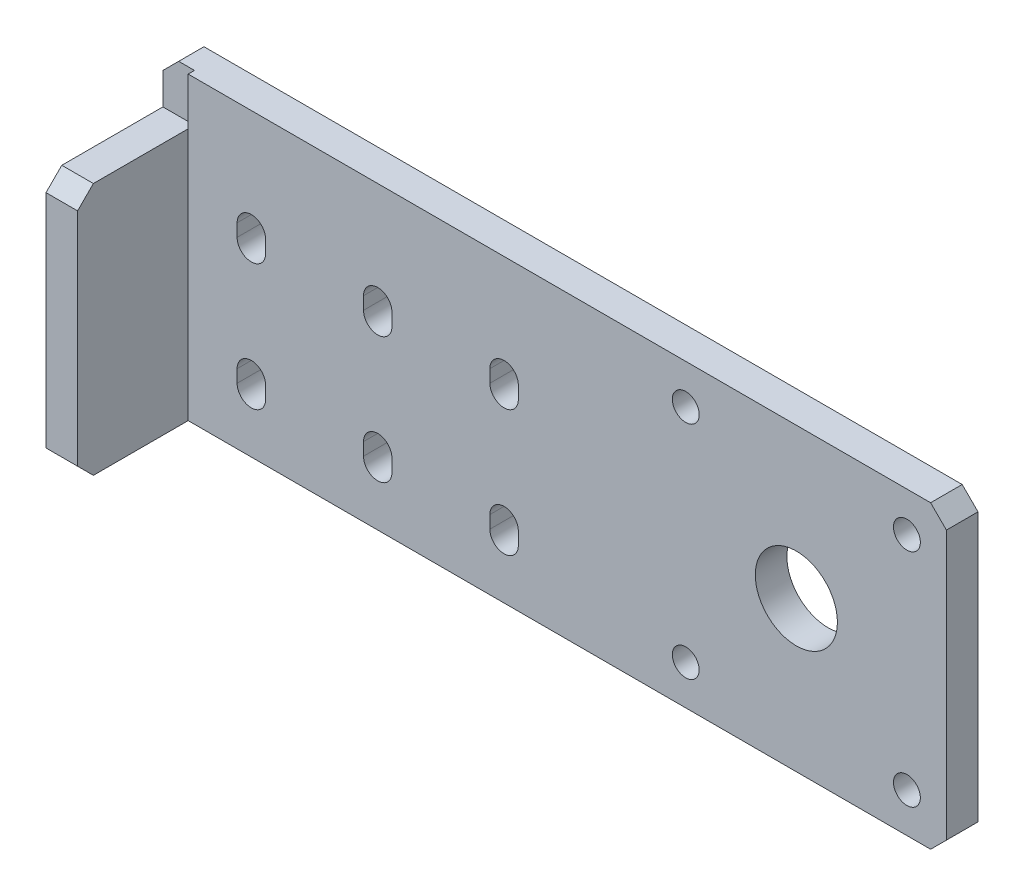
SolidWorks part; units mm, degrees
material "AISI 1045 钢，冷拔"
ref_plane "前视基准面" through (0, 0, 0) normal (0, 0, 1) x (1, 0, 0)
ref_plane "上视基准面" through (0, 0, 0) normal (0, 1, 0) x (1, 0, 0)
ref_plane "右视基准面" through (0, 0, 0) normal (1, 0, 0) x (0, 0, -1)
sketch "草图1" plane through (0, 0, 0) normal (0, 0, 1) x (1, 0, 0)
  line L1 (-125, 47.5) -> (125, 47.5)
  line L2 (-125, 47.5) -> (-125, -47.5)
  line L3 (-125, -47.5) -> (125, -47.5)
  line L4 (125, 47.5) -> (125, -47.5)
  line L5 (-125, 47.5) -> (125, -47.5) construction
  line L6 (-125, -47.5) -> (125, 47.5) construction
  point P0 (0, 0)
  dimension "D1" = 95
  dimension "D2" = 250
extrude "凸台-拉伸1" add sketch "草图1" along normal blind 10
sketch "草图3" plane through (0, 0, 10) normal (0, 0, 1) x (1, 0, 0)
  line L0 (-55, 17.5058) -> (-55, -69.5405) construction
  line L1 (125, -47.5) -> (125, 47.5) construction
  line L2 (-22.9727, -29.5) -> (-57.0867, -29.5) construction
  line L3 (-125, -47.5) -> (125, -47.5) construction
  line L4 (-55, -29.5) -> (-55, -25.5) construction
  line L5 (-59.5, -29.5) -> (-59.5, -25.5)
  line L6 (-50.5, -29.5) -> (-50.5, -25.5)
  arc A0 (-59.5, -29.5) -> (-50.5, -29.5) centre (-55, -29.5) ccw
  arc A1 (-50.5, -25.5) -> (-59.5, -25.5) centre (-55, -25.5) ccw
  point P10 (-55, -27.5)
  dimension "D4" = 4.5
  dimension "D1" = 180
  dimension "D2" = 18
  dimension "D3" = 4
extrude "切除-拉伸2" cut sketch "草图3" against normal through all
pattern_linear "阵列(线性)1" count 2 spacing 40 along (1, 0, 0) count 2 spacing 40 along (0, 1, 0) of "切除-拉伸2"
pattern_linear "阵列(线性)2" count 2 spacing 40 along (-1, 0, 0) count 2 spacing 40 along (0, 1, 0) of "切除-拉伸2"
sketch "草图10" plane through (0, 0, 10) normal (0, 0, 1) x (1, 0, 0)
  line L0 (24.75, 0) -> (-24.75, 0) construction
  line L1 (42.5, 35) -> (112.5, 35) construction
  line L2 (42.5, 35) -> (42.5, -35) construction
  line L3 (42.5, -35) -> (112.5, -35) construction
  line L4 (112.5, 35) -> (112.5, -35) construction
  line L5 (42.5, 35) -> (112.5, -35) construction
  line L6 (42.5, -35) -> (112.5, 35) construction
  line L7 (125, -47.5) -> (125, 47.5) construction
  point P0 (77.5, 0)
  dimension "D1" = 70
  dimension "D2" = 70
  dimension "D3" = 47.5
hole_wizard "M10 螺纹孔3" positions "3D草图3" profile "草图11" tap size "M10" standard "GB"
sketch3d "3D草图3"
  point P0 (42.5, 35, 10)
  point P3 (112.5, 35, 10)
  point P6 (112.5, -35, 10)
  point P9 (42.5, -35, 10)
sketch "草图11" plane through (42.5, 35, 10) normal (1, 0, 0) x (0, -1, 0)
  line L0 (0, 0) -> (0, 27.0537)
  line L1 (0, 27.0537) -> (4.25, 24.5)
  line L2 (4.25, 24.5) -> (4.25, 0)
  line L5 (4.25, 0) -> (0, 0)
  line L10 (0, 27.0537) -> (-4.25, 24.5) construction
  line L11 (0, -6.35) -> (0, 107.95) construction
  dimension "螺纹孔钻头直径" = 8.5
  dimension "螺纹孔钻头深度" = 24.5
  dimension "导头角度" = 118
cosmetic thread "孔螺蚊线9"
cosmetic thread "孔螺蚊线10"
cosmetic thread "孔螺蚊线11"
cosmetic thread "孔螺蚊线12"
sketch "草图12" plane through (0, 0, 10) normal (0, 0, 1) x (1, 0, 0)
  line L0 (42.5, 35) -> (112.5, -35) construction
  circle A0 centre (77.5, 0) radius 13
  dimension "D1" = 26
extrude "切除-拉伸5" cut sketch "草图12" against normal through all
sketch "草图13" plane through (0, 0, 0) normal (0, 0, -1) x (-1, 0, 0)
  line L0 (-45, -20) -> (-110, -20) construction
  line L1 (-110, -20) -> (-110, 20) construction
  line L2 (-110, 20) -> (-45, 20) construction
hole_wizard "M6 螺纹孔1" positions "3D草图4" profile "草图14" tap size "M6" standard "GB"
sketch3d "3D草图4"
  point P0 (45, -20, 0)
  point P3 (110, -20, 0)
  point P6 (110, 20, 0)
  point P9 (45, 20, 0)
sketch "草图14" plane through (45, -20, 0) normal (1, 0, 0) x (0, 1, 0)
  line L0 (0, 0) -> (0, 10)
  line L1 (0, 10) -> (2.5, 10)
  line L2 (2.5, 10) -> (2.5, 0)
  line L5 (2.5, 0) -> (0, 0)
  line L11 (0, -6.35) -> (0, 107.95) construction
  dimension "通孔螺纹孔钻头直径" = 5
  dimension "通孔螺纹孔钻头深度" = 10
cosmetic thread "孔螺蚊线17" [suppressed]
cosmetic thread "孔螺蚊线18" [suppressed]
cosmetic thread "孔螺蚊线19" [suppressed]
cosmetic thread "孔螺蚊线20" [suppressed]
sketch "草图15" plane through (-125, 0, 0) normal (-1, 0, 0) x (0, 0, 1)
  line L0 (5, -37.5) -> (5, -17.5) construction
  line L1 (5, -17.5) -> (5, 2.5) construction
  line L2 (5, 2.5) -> (5, 22.5) construction
hole_wizard "M6 螺纹孔2" positions "3D草图5" profile "草图16" tap size "M6" standard "GB"
sketch3d "3D草图5"
  point P0 (-125, -37.5, 5)
  point P3 (-125, -17.5, 5)
  point P6 (-125, 2.5, 5)
  point P9 (-125, 22.5, 5)
sketch "草图16" plane through (-125, -37.5, 5) normal (0, 1, 0) x (0, 0, 1)
  line L0 (0, 0) -> (0, 16.5022)
  line L1 (0, 16.5022) -> (2.5, 15)
  line L2 (2.5, 15) -> (2.5, 0)
  line L5 (2.5, 0) -> (0, 0)
  line L10 (0, 16.5022) -> (-2.5, 15) construction
  line L11 (0, -6.35) -> (0, 107.95) construction
  dimension "螺纹孔钻头直径" = 5
  dimension "螺纹孔钻头深度" = 15
  dimension "导头角度" = 118
cosmetic thread "孔螺蚊线21" [suppressed]
cosmetic thread "孔螺蚊线22" [suppressed]
cosmetic thread "孔螺蚊线23" [suppressed]
cosmetic thread "孔螺蚊线24" [suppressed]
sketch "草图18" plane through (0, -47.5, 0) normal (0, -1, 0) x (1, 0, 0)
  line L0 (12, 5) -> (47, 5) construction
  line L1 (47, 5) -> (82, 5) construction
  line L2 (82, 5) -> (117, 5) construction
  point P4 (64.5, 5)
hole_wizard "M4 螺纹孔1" positions "3D草图6" profile "草图19" tap size "M4" standard "GB"
sketch3d "3D草图6"
  point P0 (117, -47.5, 5)
  point P9 (12, -47.5, 5)
  point P12 (64.5, -47.5, 5)
sketch "草图19" plane through (117, -47.5, 5) normal (1, 0, 0) x (0, 0, -1)
  line L0 (0, 0) -> (0, 11.0914)
  line L1 (0, 11.0914) -> (1.65, 10.1)
  line L2 (1.65, 10.1) -> (1.65, 0)
  line L5 (1.65, 0) -> (0, 0)
  line L10 (0, 11.0914) -> (-1.65, 10.1) construction
  line L11 (0, -6.35) -> (0, 107.95) construction
  dimension "螺纹孔钻头直径" = 3.3
  dimension "螺纹孔钻头深度" = 10.1
  dimension "导头角度" = 118
cosmetic thread "孔螺蚊线25"
cosmetic thread "孔螺蚊线26"
cosmetic thread "孔螺蚊线28"
sketch "草图22" plane through (0, 0, 10) normal (0, 0, 1) x (1, 0, 0)
  line L0 (-125, -47.5) -> (125, -47.5) construction
  line L1 (-125, 47.5) -> (-115, 47.5)
  line L2 (-125, 47.5) -> (-125, -47.5)
  line L3 (-125, -47.5) -> (-115, -47.5)
  line L4 (-115, 47.5) -> (-115, -47.5)
  dimension "D1" = 10
extrude "切除-拉伸6" cut sketch "草图22" against normal blind 2
sketch "草图21" plane through (0, 0, 8) normal (0, 0, -1) x (-1, 0, 0)
  line L1 (125, -47.5) -> (115, -47.5)
  line L2 (125, -47.5) -> (125, 32.5)
  line L3 (125, 32.5) -> (115, 32.5)
  line L4 (115, -47.5) -> (115, 32.5)
  dimension "D1" = 80
  dimension "D2" = 10
extrude "凸台-拉伸2" add sketch "草图21" against normal blind 37 separate body
chamfer "倒角1" distance 5 angle 45 3 edges at (125, -47.5, 5) (125, 47.5, 5) (-125, 47.5, 4)
chamfer "倒角2" distance 5 angle 45 2 edges at (-120, 32.5, 45) (-120, -47.5, 45)
